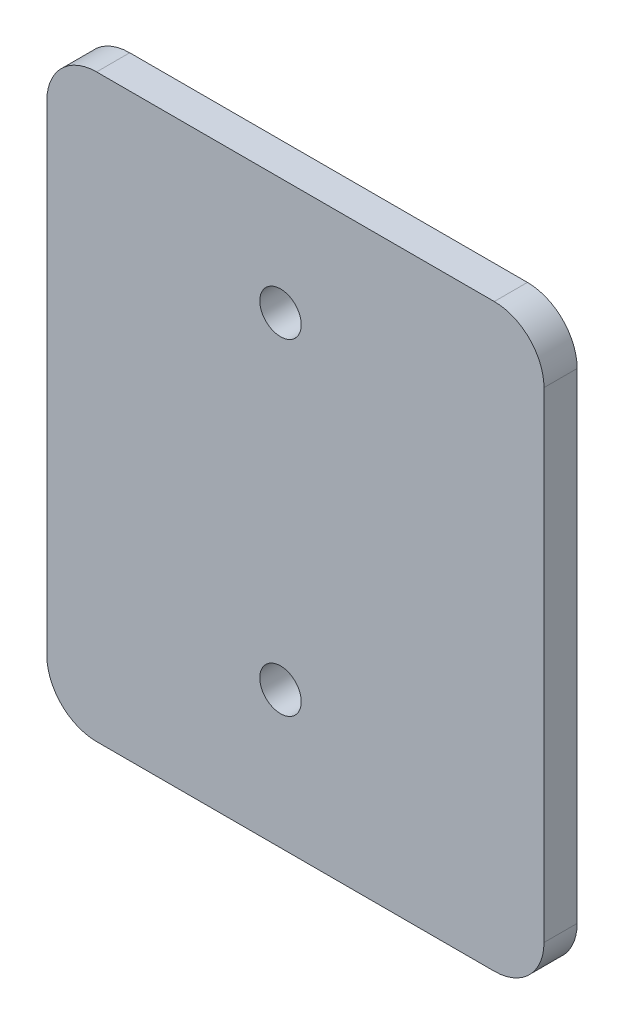
SolidWorks part; units mm, degrees
ref_plane "Front Plane" through (0, 0, 0) normal (0, 0, 1) x (1, 0, 0)
ref_plane "Top Plane" through (0, 0, 0) normal (0, 1, 0) x (1, 0, 0)
ref_plane "Right Plane" through (0, 0, 0) normal (1, 0, 0) x (0, 0, -1)
other "Configuration Table"
sketch "Sketch1" plane through (0, 0, 0) normal (0, 0, 1) x (1, 0, 0)
  line L0 (-87.2895, 24.845) -> (-87.2895, -359.155) construction
  line L1 (-87.2895, -33.155) -> (-57.2895, -33.155)
  line L2 (-87.2895, -33.155) -> (-87.2895, -68.155)
  line L3 (-87.2895, -68.155) -> (-57.2895, -68.155)
  line L4 (-57.2895, -33.155) -> (-57.2895, -68.155)
  line L5 (17.7105, 36.845) -> (-86.2895, 36.845) construction
  dimension "D1" = 35
  dimension "D2" = 30
  dimension "D3" = 70
extrude "Boss-Extrude1" add sketch "Sketch1" along normal blind 2
fillet "Fillet1" radius 3 4 edges at (-57.2895, -68.155, 1) (-57.2895, -33.155, 1) (-87.2895, -33.155, 1) (-87.2895, -68.155, 1)
hole_wizard "M3 Tapped Hole1" positions "Sketch2" profile "Sketch3" tap size "M3" standard "GB" end condition through all
sketch "Sketch2" plane through (0, 0, 2) normal (0, 0, 1) x (1, 0, 0)
  line L0 (-71.5895, -40.1944) -> (-87.2895, -40.1944) construction
  line L1 (-71.5895, -39.6444) -> (-71.5895, -40.7444) construction
  line L2 (-87.2895, -36.155) -> (-87.2895, -65.155) construction
  line L4 (-71.5895, -59.8944) -> (-87.2895, -59.8944) construction
  line L5 (-71.5895, -59.3444) -> (-71.5895, -60.4444) construction
  line L7 (-73.1895, -63.0444) -> (-73.1895, -33.155) construction
  line L8 (-70.0895, -63.0444) -> (-76.2895, -63.0444) construction
  line L9 (-60.2895, -33.155) -> (-84.2895, -33.155) construction
  point P33 (-73.1895, -40.1944)
  point P35 (-73.1895, -59.8944)
sketch "Sketch3" plane through (-73.1895, -59.8944, 2) normal (1, 0, 0) x (0, -1, 0)
  line L0 (0, 0) -> (0, 2)
  line L1 (0, 2) -> (1.25, 2)
  line L2 (1.25, 2) -> (1.25, 0)
  line L5 (1.25, 0) -> (0, 0)
  line L11 (0, -6.35) -> (0, 107.95) construction
  dimension "通孔螺纹孔钻头直径" = 2.5
  dimension "通孔螺纹孔钻头深度" = 2
cosmetic thread "Hole thread line1" parameters "D2"=3
cosmetic thread "Hole thread line2" parameters "D2"=3
